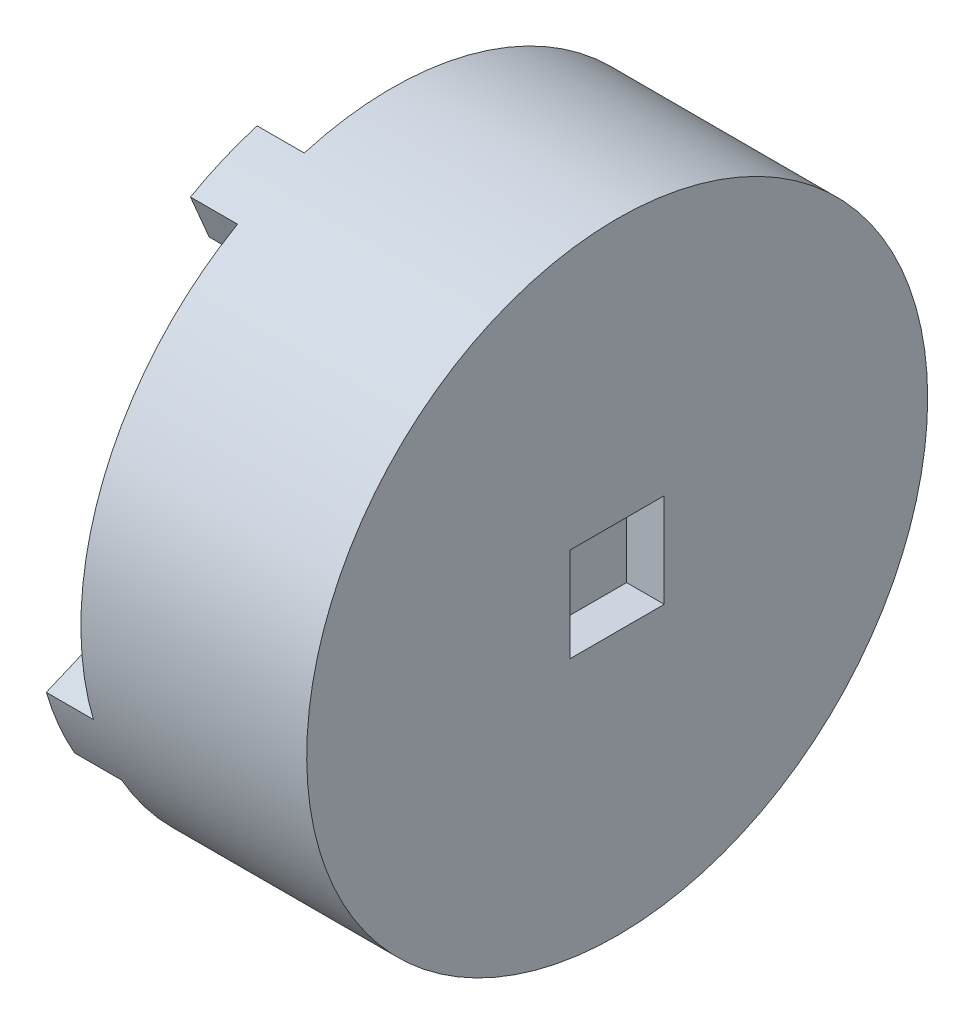
from build123d import *

# Parameters (mm, degrees)
SKETCH_1_R               = 16.5
EXTRUDE_1_DEPTH          = 12
SKETCH_2_R               = 3.75
CUT_EXTRUDE_1_DEPTH      = 4
EXTRUDE_START            = 2.5
EXTRUDE_2_DEPTH          = 2.5
PATTERN_CIRCULAR_1_COUNT = 4
SKETCH_4_R               = 2.25
SKETCH_4_R_2             = 2
CUT_EXTRUDE_2_DEPTH      = 4
SKETCH_5_W               = 5
SKETCH_5_H               = 5
CUT_EXTRUDE_3_DEPTH      = 2


with BuildPart() as part:
    # 草图1 → 凸台-拉伸1 (new body)
    with BuildSketch(Plane(origin=(0, 0, 0), x_dir=(0, 0, -1), z_dir=(1, 0, 0))):
        Circle(SKETCH_1_R)
    extrude(amount=EXTRUDE_1_DEPTH)

    # 草图2 → 切除-拉伸1 (cut)
    with BuildSketch(Plane.ZY):
        Circle(SKETCH_2_R)
    extrude(amount=-CUT_EXTRUDE_1_DEPTH, mode=Mode.SUBTRACT)

    # 草图3 → 凸台-拉伸2 (add)
    with BuildSketch(Plane.ZY.offset(EXTRUDE_START)):
        with BuildLine():
            Line((-3.639654287, -13.501149643), (-4.631065603, -15.836768338))
            ThreePointArc((-4.631065603, -15.836768338), (-6.44706362, -15.188330082), (-8.175009289, -14.332453493))
            Line((-8.175009289, -14.332453493), (-7.183597972, -11.996834798))
            Line((-7.183597972, -11.996834798), (-3.639654287, -13.501149643))
        make_face()
    extrude_2 = extrude(amount=-EXTRUDE_2_DEPTH)

    # 阵列(圆周)1: 凸台-拉伸2 ×4 about axis
    pattern_circular_1_axis = Axis((0, 0, 0), (1, 0, 0))
    for i in range(1, PATTERN_CIRCULAR_1_COUNT):
        add(extrude_2.rotate(pattern_circular_1_axis, i * 360 / PATTERN_CIRCULAR_1_COUNT))

    # 草图4 → 切除-拉伸2 (cut)
    with BuildSketch(Plane.ZY):
        with Locations((-1.282674839, 10.446548246)):
            Circle(SKETCH_4_R)
        with Locations((1.282674839, -10.446548246)):
            Circle(SKETCH_4_R_2)
    extrude(amount=-CUT_EXTRUDE_2_DEPTH, mode=Mode.SUBTRACT)

    # 草图5 → 切除-拉伸3 (cut)
    with BuildSketch(Plane(origin=(12, 0, 0), x_dir=(0, 0, -1), z_dir=(1, 0, 0))):
        Rectangle(SKETCH_5_W, SKETCH_5_H)
    extrude(amount=-CUT_EXTRUDE_3_DEPTH, mode=Mode.SUBTRACT)


solid = part.part
